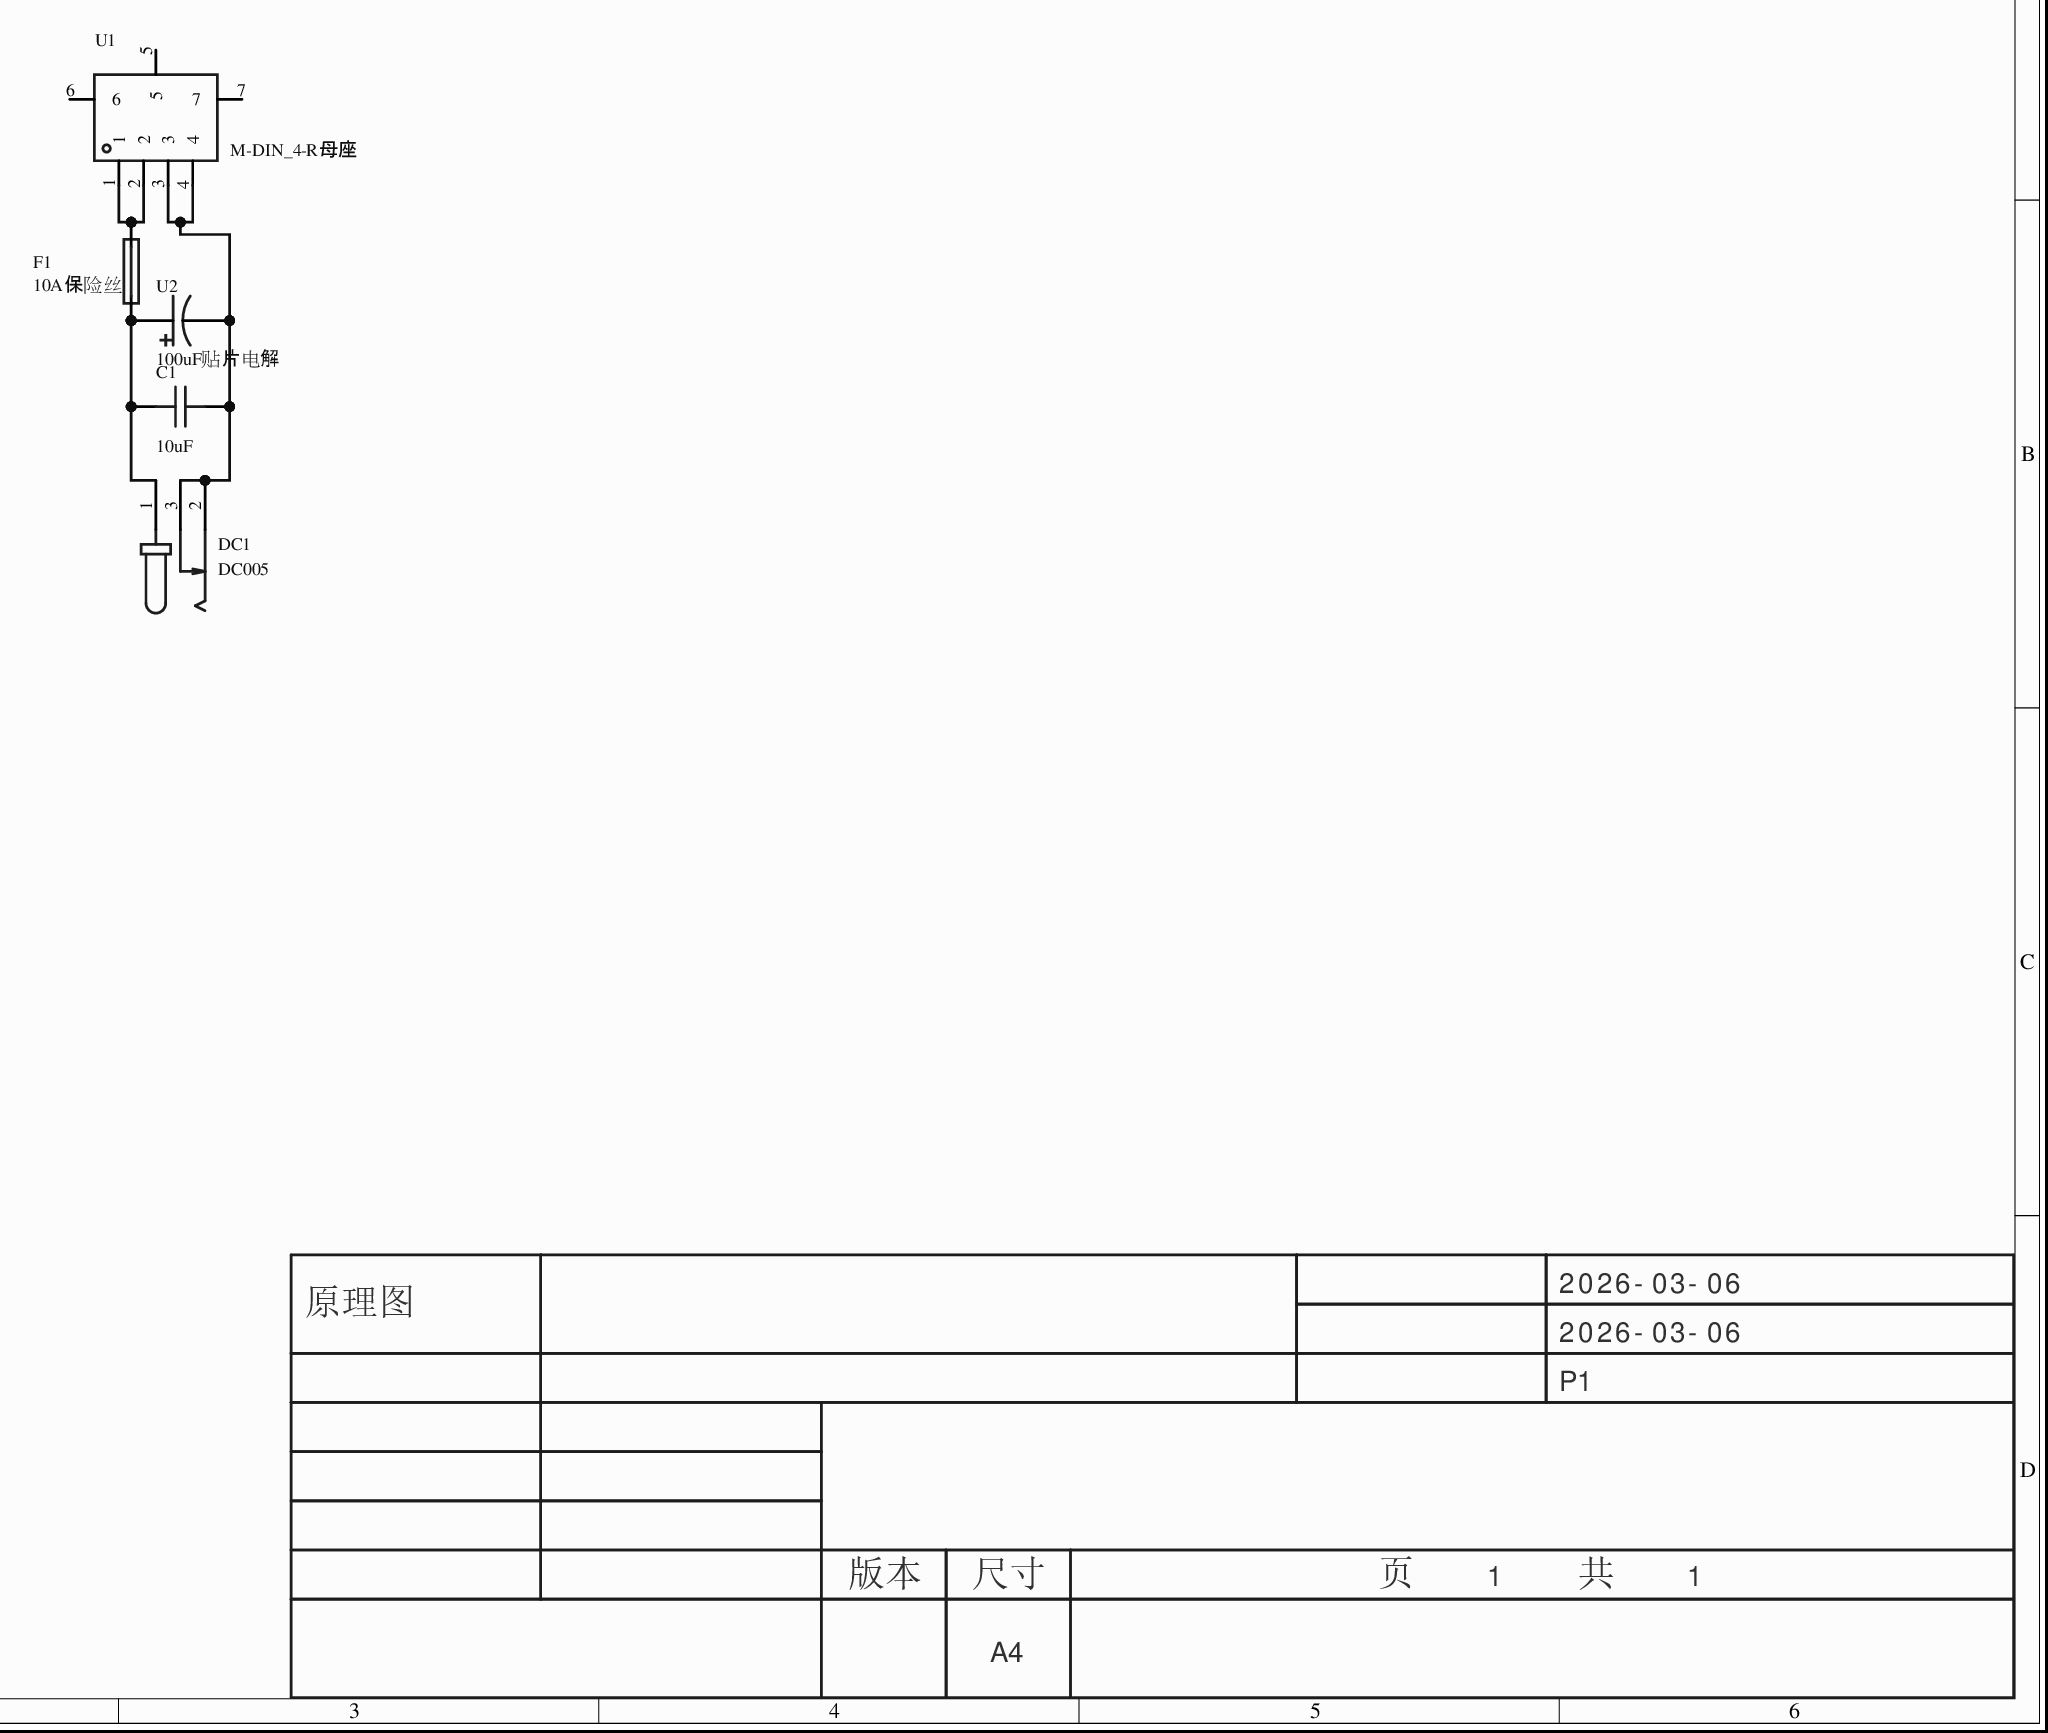
[diagram p0: MISC51882-3.schdoc]
# Altium project MISC51882-2.PrjPcb
1 sheet, 5 parts. Net scope: global (net labels, ports and power ports of the same name join across sheets).
Board file: MISC51882.pcbdoc

## Sheet MISC51882-3.schdoc
size 297 x 209 mm; Version: V1.0; @Project Name: MISC51882; @Update Date: 2026-03-06; @Create Date: 2026-03-06; @Board Name: MISC51882; @Create Time: 17:23:38; @Page Count: 1; @Page No: 1; @Schematic Name: MISC51882; @Update Time: 17:23:38; Size: A4

### Parts
C1  10uF  [C0603]
DC1  DC005  [DC-IN-TH_DC005]
F1  10A保险丝  [FUSE-SMD_L6.1-W2.6]
U1  M-DIN_4-R母座  [CONN-TH_DIN_4P_12D8]
U2  100uF贴片电解  [CAP-SMD_BD6.3-L6.6-W6.6-LS7.4-FD]

### Nets
NetC1_1: C1.1 DC1.1 F1.1 U2.1
NetC1_2: C1.2 DC1.2 DC1.3 U1.3 U1.4 U2.2
NetF1_2: F1.2 U1.1 U1.2

Not connected (* = marked no-connect by the designer): U1 5 6 7

### Notes on the sheet
- 2026-03-06
- 原理图
- P1
- 版本
- 尺寸
- A4
- 页    1    共    1

### Library data of the parts
C1 = CAP_0603: Symbol: Capacitance; ConvertToPcb: yes; ModelId: ac125912035d415993ca9572d50418b10819f05c4eef4c71ace90d822a990e87; ModelName: C0603_L1.6-W0.8-H0.8; ModelTransform: 62.992,31.496,0,0,0,0,0,0,0; Device: CAP_0603; Value: 10uF; AddInBom: yes; Supplier Footprint: 0603; FootprintName: C0603
DC1 = DC005: 连接器类型:DC电源插座;安装方式:弯插;触点内径:2mm;触点外径:6.3mm;额定电流:500mA;额定电压:12V;工作温度:-30℃~+70℃;; Manufacturer: SHOU HAN(首韩); Symbol: DC005_C431533; AddInBom: yes; ModelId: f168fe383f964e0ea2af0127ff6ac7b40819f05c4eef4c71ace90d822a990e87; ModelTransform: 366.141,553.149,0,270,0,0,-141.734,88.583,-149.606; Connector Type: DC电源插座; Inside Contact Diameter: 2mm; Outside Contact Diameter: 6.3mm; Current Rating: 500mA; Voltage Rating (Max): 12V; Device: DC005; LCSC Part Name: DC005-2.0 黑（铁）; SupplierPart: C431533; ManufacturerPart: DC005; Supplier Footprint: 插件; JLCPCB Part Class: Extended Part; Datasheet: https://item.szlcsc.com/datasheet/DC005/427890.html; Supplier: LCSC; ConvertToPcb: yes; FootprintName: DC-IN-TH_DC005; ModelName: DC-IN-TH_DC005; Mounting Type: 弯插; Operating Temperature: -30℃~+70℃
F1 = 10A保险丝: AddInBom: yes; ModelId: 8dc97aad3e5d43c2b990fd56287574220819f05c4eef4c71ace90d822a990e87; ModelName: FUSE-SMD_L6.1-W2.6-H2.6; ModelTransform: 240.157,102.362,0,0,0,0,0,0,0; Symbol: 10A保险丝; Device: 10A保险丝; LCSC Part Name: 10A保险丝; SupplierPart: C9900011494; ManufacturerPart: 10A保险丝; Supplier Footprint: 1808; JLCPCB Part Class: Extended Part; Supplier: LCSC; ConvertToPcb: yes; FootprintName: FUSE-SMD_L6.1-W2.6
U1 = M-DIN_4-R母座: AddInBom: yes; ModelId: 054c353fa19d4ee3ace38fdba3592bb60819f05c4eef4c71ace90d822a990e87; ModelTransform: 551.5737,507.873,0,180,0,0,0,65,-157.48; Symbol: M-DIN_4-R母座; Device: M-DIN_4-R母座; LCSC Part Name: M-DIN_4-R母座; SupplierPart: C9900011966; ManufacturerPart: M-DIN_4-R母座; Supplier Footprint: DIN_4P_12D8; JLCPCB Part Class: Extended Part; Supplier: LCSC; ConvertToPcb: yes; FootprintName: CONN-TH_DIN_4P_12D8; ModelName: CONN-TH_DIN_4P_12D8
U2 = 100uF贴片电解: AddInBom: yes; ModelId: 1416614ffc1f4b92814ec0fcf834cf2d0819f05c4eef4c71ace90d822a990e87; ModelTransform: 291.338,259.842,0,180,0,0,-0.004,-0.007,0; Symbol: 100UF贴片电解; Device: 100uF贴片电解; LCSC Part Name: 100uF贴片电解; SupplierPart: C9900002196; ManufacturerPart: 100uF贴片电解; Supplier Footprint: 100uF; JLCPCB Part Class: Extended Part; Supplier: LCSC; ConvertToPcb: yes; FootprintName: CAP-SMD_BD6.3-L6.6-W6.6-LS7.4-FD; ModelName: CAP-SMD_BD6.3-L6.6-W6.6-LS7.4-FD